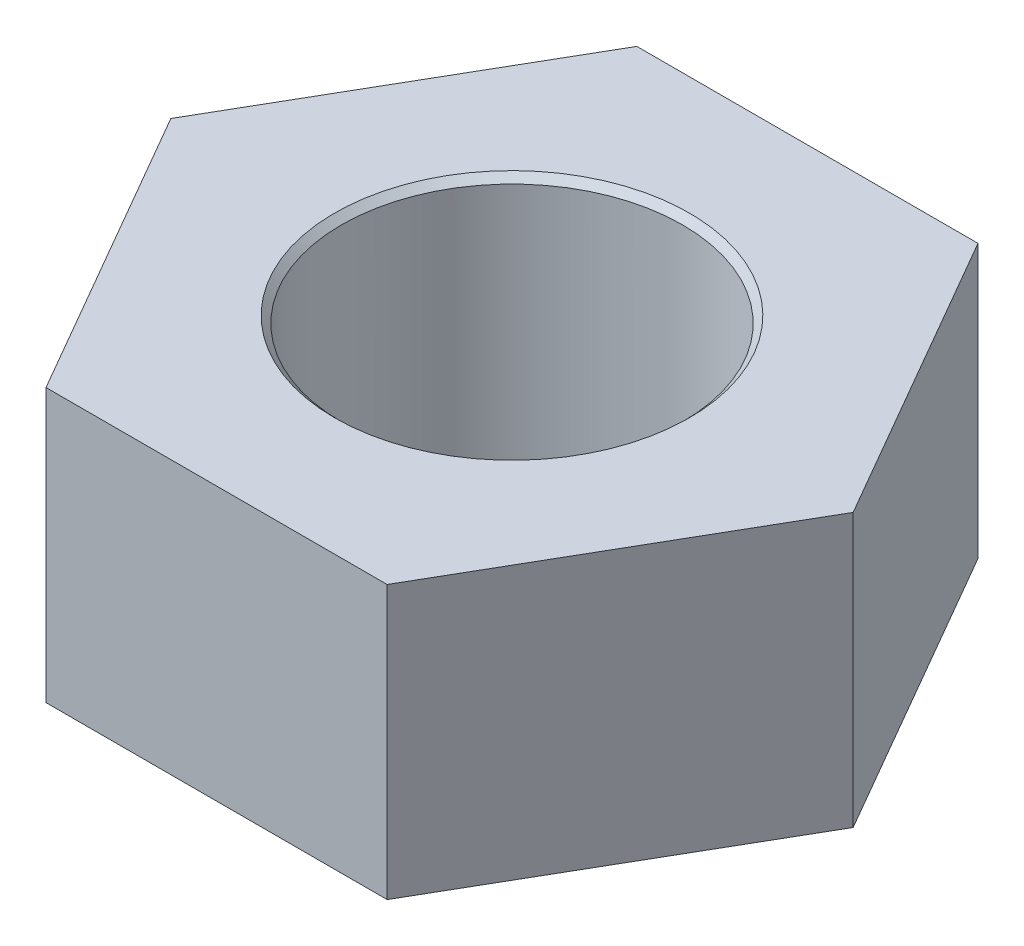
SolidWorks part; units mm, degrees
ref_plane "Front Plane" through (0, 0, 0) normal (0, 0, 1) x (1, 0, 0)
ref_plane "Top Plane" through (0, 0, 0) normal (0, 1, 0) x (1, 0, 0)
ref_plane "Right Plane" through (0, 0, 0) normal (1, 0, 0) x (0, 0, -1)
other "Configuration Table"
sketch "Sketch1" plane through (0, 0, 0) normal (0, 1, 0) x (1, 0, 0)
  line L1 (2.5, -4.3301) -> (5, 0)
  line L2 (5, 0) -> (2.5, 4.3301)
  line L3 (2.5, 4.3301) -> (-2.5, 4.3301)
  line L4 (-2.5, 4.3301) -> (-5, 0)
  line L5 (-5, 0) -> (-2.5, -4.3301)
  line L6 (-2.5, -4.3301) -> (2.5, -4.3301)
  circle A0 centre (0, 0) radius 2.5
  circle A1 centre (0, 0) radius 4.3301 construction
  point P3 (0, 4.3301)
  dimension "D1" = 5
  dimension "D2" = 5
extrude "Boss-Extrude1" add sketch "Sketch1" along normal blind 4
chamfer "Chamfer1" distance 0.1 angle 45 2 edges at (0, 0, 2.5) (0, 4, 2.5)
